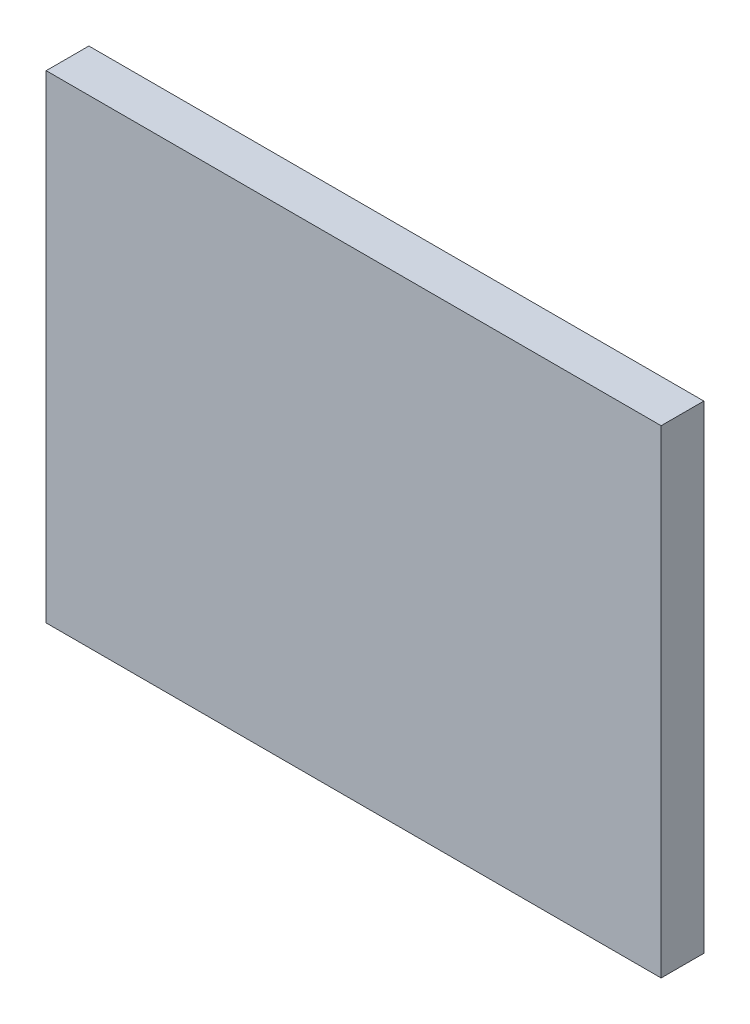
SolidWorks part; units mm, degrees
ref_plane "前视基准面" through (0, 0, 0) normal (0, 0, 1) x (1, 0, 0)
ref_plane "上视基准面" through (0, 0, 0) normal (0, 1, 0) x (1, 0, 0)
ref_plane "右视基准面" through (0, 0, 0) normal (1, 0, 0) x (0, 0, -1)
sketch "草图1" plane through (0, 0, 0) normal (0, 0, 1) x (1, 0, 0)
  line L1 (-180, 140) -> (180, 140)
  line L2 (-180, 140) -> (-180, -140)
  line L3 (-180, -140) -> (180, -140)
  line L4 (180, 140) -> (180, -140)
  line L5 (-180, 140) -> (180, -140) construction
  line L6 (-180, -140) -> (180, 140) construction
  point P0 (0, 0)
  dimension "D1" = 360
  dimension "D2" = 280
extrude "凸台-拉伸1" add sketch "草图1" along normal blind 25
